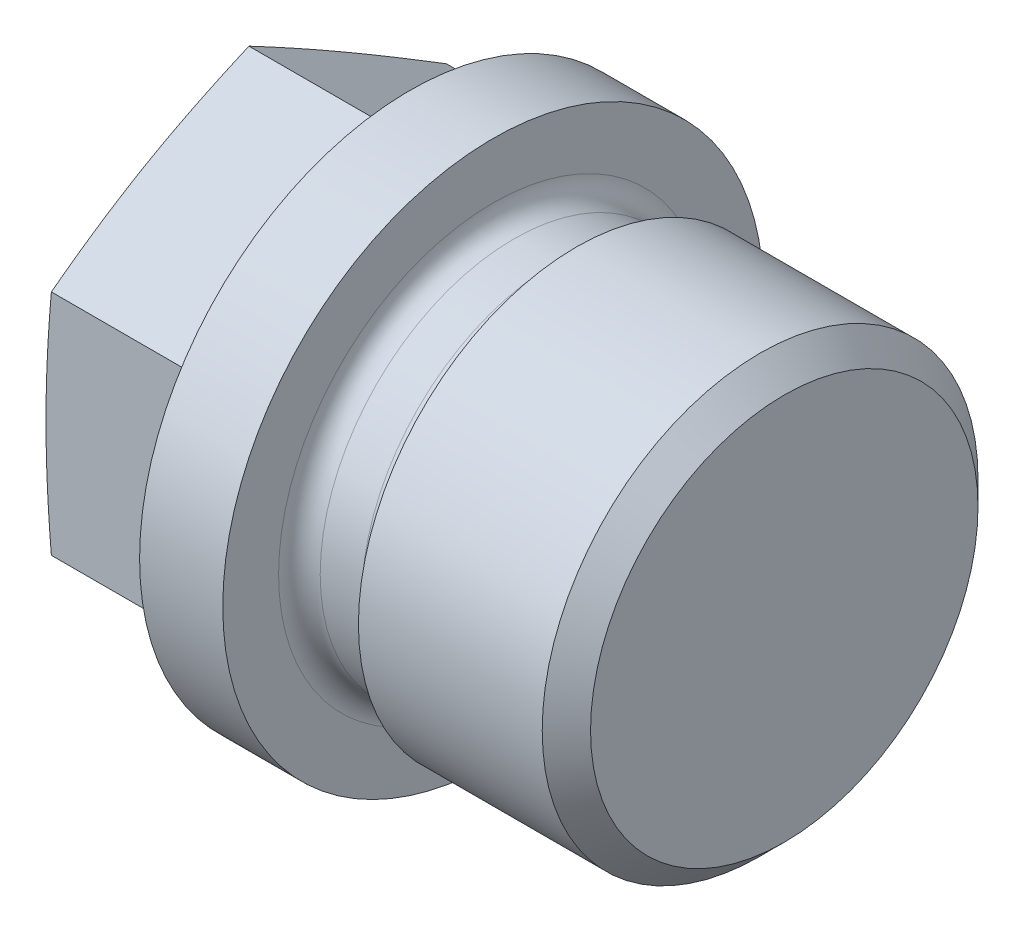
SolidWorks part; units mm, degrees
material "35钢"
ref_plane "Front Plane" through (0, 0, 0) normal (0, 0, 1) x (1, 0, 0)
ref_plane "Top Plane" through (0, 0, 0) normal (0, 1, 0) x (1, 0, 0)
ref_plane "Right Plane" through (0, 0, 0) normal (1, 0, 0) x (0, 0, -1)
sketch "Sketch1" plane through (0, 0, 0) normal (0, 0, 1) x (1, 0, 0)
  line L0 (0, 0) -> (26, 0) construction
  line L1 (26, 0) -> (26, 10.4775) construction
  line L2 (26, 10.4775) -> (16, 10.4775) construction
  line L3 (16, 10.4775) -> (16, 9.3155)
  line L4 (16, 9.3155) -> (12, 9.3155)
  line L5 (12, 9.3155) -> (12, 13)
  line L6 (12, 13) -> (8, 13)
  line L7 (8, 13) -> (8, 1.5)
  line L8 (8, 1.5) -> (0, 1.5)
  line L9 (0, 1.5) -> (0, 0)
  line L10 (0, 0) -> (26, 0)
  line L11 (24.838, 10.4775) -> (26, 9.3155)
  line L12 (16, 10.4775) -> (24.838, 10.4775)
  line L13 (26, 9.3155) -> (26, 0)
  dimension "L" = 26
  dimension "b" = 4
  dimension "1" = 14
  dimension "d" = 20.955
  dimension "Do" = 26
  dimension "D6" = 3
  dimension "d1" = 18.631
  dimension "D8" = 45
revolve "Revolve1" add sketch "Sketch1" angle 360 about L0
sketch "Sketch2" plane through (0, 0, 0) normal (-1, 0, 0) x (0, 0, 1)
  line L1 (0, 10.9697) -> (-9.5, 5.4848)
  line L2 (-9.5, 5.4848) -> (-9.5, -5.4848)
  line L3 (-9.5, -5.4848) -> (0, -10.9697)
  line L4 (0, -10.9697) -> (9.5, -5.4848)
  line L5 (9.5, -5.4848) -> (9.5, 5.4848)
  line L6 (9.5, 5.4848) -> (0, 10.9697)
  circle A0 centre (0, 0) radius 9.5 construction
  dimension "s" = 19
extrude "Extrude1" add sketch "Sketch2" against normal up to surface (8 mm away) up to face at (8, 0, 1.5)
sketch "Sketch3" plane through (0, 0, 0) normal (-1, 0, 0) x (0, 0, 1)
  circle A0 centre (0, 0) radius 9.5 construction
  circle A1 centre (0, 0) radius 9.5
extrude "Cut-Extrude1" cut sketch "Sketch3" against normal blind 10 draft 80 flip side to cut
fillet "Fillet1" radius 1 2 edges at (16, 0, 9.3155) (12, 0, 9.3155)
